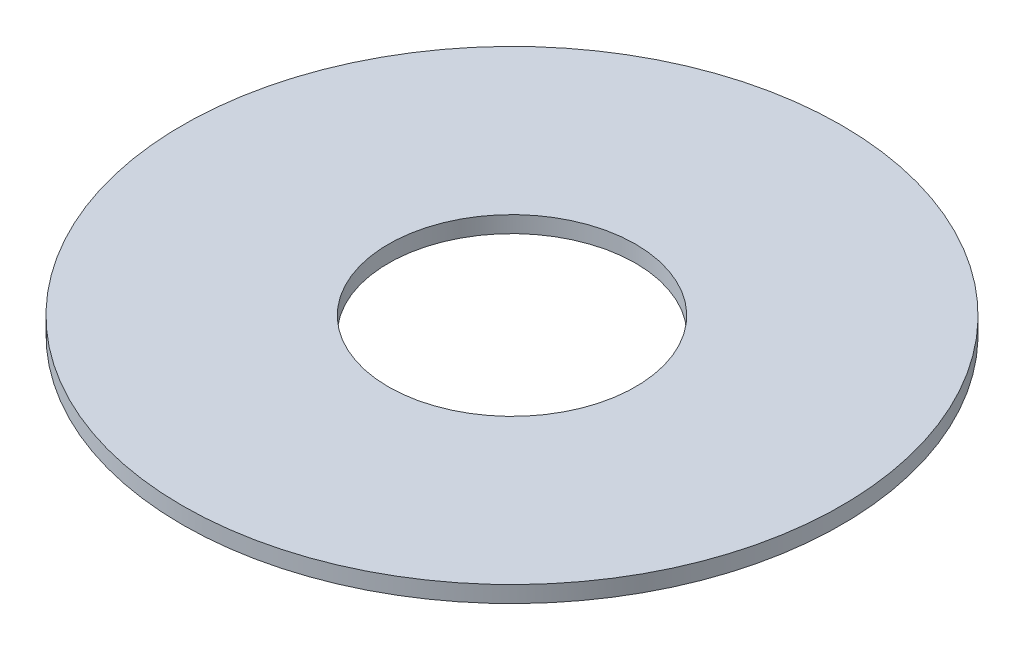
from build123d import *

# Parameters (mm, degrees)
SKETCH1_R           = 60
SKETCH1_R_2         = 22.5
BOSS_EXTRUDE1_DEPTH = 3


with BuildPart() as part:
    # Sketch1 → Boss-Extrude1 (new body)
    with BuildSketch(Plane(origin=(0, 0, 0), x_dir=(1, 0, 0), z_dir=(0, 1, 0))):
        with Locations(Location((0, 0, 0), (0, 0, 270))):
            Circle(SKETCH1_R)
        with Locations(Location((0, 0, 0), (0, 0, 270))):
            Circle(SKETCH1_R_2, mode=Mode.SUBTRACT)
    extrude(amount=BOSS_EXTRUDE1_DEPTH)


solid = part.part
